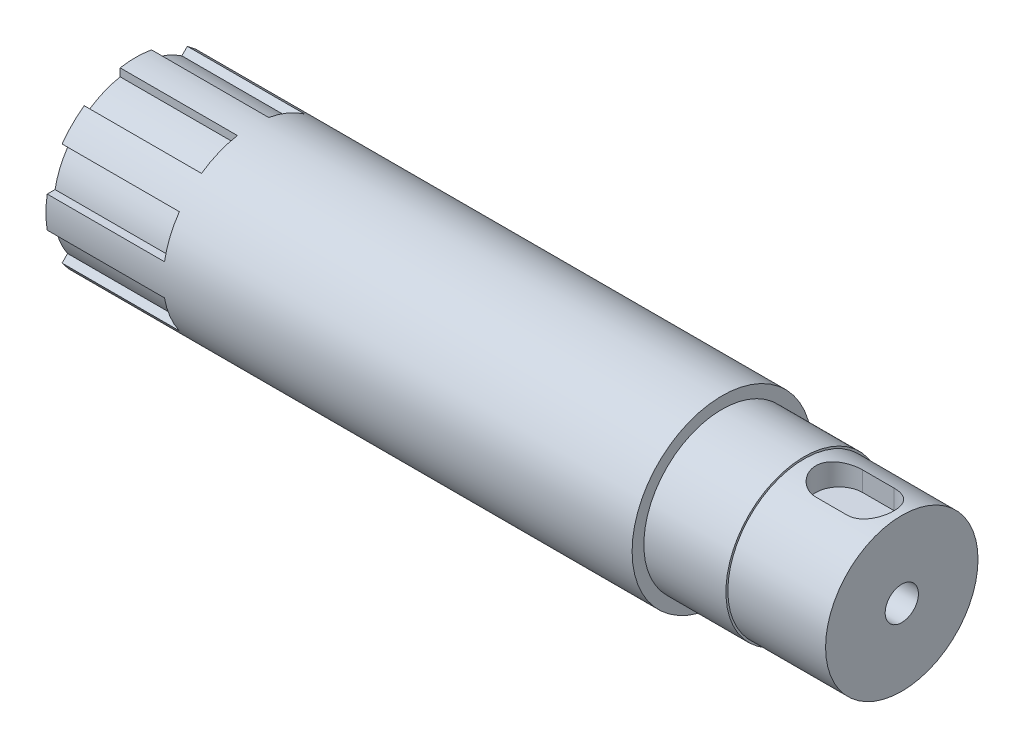
from build123d import *

# Parameters (mm, degrees)
SKETCH_1_R              = 19.5
EXTRUDE_1_DEPTH         = 25
CUT_EXTRUDE_1_DEPTH     = 5.95
SKETCH_3_R              = 20
EXTRUDE_2_DEPTH         = 21
SKETCH_4_R              = 23
EXTRUDE_3_DEPTH         = 150
CUT_EXTRUDE_START       = -30
CUT_EXTRUDE_2_DEPTH     = 30
HOLE_WIZARD_M10_1_D     = 8.5
HOLE_WIZARD_M10_1_DEPTH = 20
HOLE_WIZARD_M10_1_TIP   = 2.553657631


with BuildPart() as part:
    # 草图1 → 凸台-拉伸1 (new body)
    with BuildSketch(Plane(origin=(0, 0, 0), x_dir=(0, 0, -1), z_dir=(1, 0, 0))):
        Circle(SKETCH_1_R)
    extrude(amount=EXTRUDE_1_DEPTH)

    # 草图2 → 切除-拉伸1 (cut)
    with BuildSketch(Plane(origin=(0, 19.5, 0), x_dir=(1, 0, 0), z_dir=(0, 1, 0))):
        with BuildLine():
            Line((9, 6), (17, 6))
            ThreePointArc((17, 6), (23, 0), (17, -6))
            Line((17, -6), (9, -6))
            ThreePointArc((9, -6), (3, 0), (9, 6))
        make_face()
    extrude(amount=-CUT_EXTRUDE_1_DEPTH, mode=Mode.SUBTRACT)

    # 草图3 → 凸台-拉伸2 (add)
    with BuildSketch(Plane.ZY):
        with Locations(Location((0, 0, 0), (0, 0, 180))):
            Circle(SKETCH_3_R)
    extrude(amount=EXTRUDE_2_DEPTH)

    # 草图4 → 凸台-拉伸3 (add)
    with BuildSketch(Plane.ZY.offset(21)):
        Circle(SKETCH_4_R)
    extrude(amount=EXTRUDE_3_DEPTH)

    # 草图5 → 切除-拉伸2 (cut)
    with BuildSketch(Plane.ZY.offset(171).offset(CUT_EXTRUDE_START)):
        with BuildLine():
            ThreePointArc((18.852862485, -13.174580681), (21.255112475, -8.78750213), (22.652173913, -3.98484843))
            Line((22.652173913, -3.98484843), (20.658042319, -3.98484843))
            ThreePointArc((20.658042319, -3.98484843), (19.443275073, -8.036963599), (17.442433123, -11.764151318))
            Line((17.442433123, -11.764151318), (18.852862485, -13.174580681))
        make_face()
        with BuildLine():
            ThreePointArc((22.646822247, 4.01515157), (21.243336512, 8.81593182), (18.83521913, 13.199792435))
            Line((18.83521913, 13.199792435), (17.425155157, 11.789728463))
            ThreePointArc((17.425155157, 11.789728463), (19.431463114, 8.065480192), (20.652173913, 4.01515157))
            Line((20.652173913, 4.01515157), (22.646822247, 4.01515157))
        make_face()
        with BuildLine():
            Line((-20.652173913, -4.01515157), (-22.646822247, -4.01515157))
            ThreePointArc((-22.646822247, -4.01515157), (-21.243336512, -8.81593182), (-18.83521913, -13.199792435))
            Line((-18.83521913, -13.199792435), (-17.425155157, -11.789728463))
            ThreePointArc((-17.425155157, -11.789728463), (-19.431463114, -8.065480192), (-20.652173913, -4.01515157))
        make_face()
        with BuildLine():
            Line((-11.764151318, -17.442433123), (-13.174580681, -18.852862485))
            ThreePointArc((-13.174580681, -18.852862485), (-8.78750213, -21.255112475), (-3.98484843, -22.652173913))
            Line((-3.98484843, -22.652173913), (-3.98484843, -20.658042319))
            ThreePointArc((-3.98484843, -20.658042319), (-8.036963599, -19.443275073), (-11.764151318, -17.442433123))
        make_face()
        with BuildLine():
            ThreePointArc((4.01515157, -22.646822247), (8.81593182, -21.243336512), (13.199792435, -18.83521913))
            Line((13.199792435, -18.83521913), (11.789728463, -17.425155157))
            ThreePointArc((11.789728463, -17.425155157), (8.065480192, -19.431463114), (4.01515157, -20.652173913))
            Line((4.01515157, -20.652173913), (4.01515157, -22.646822247))
        make_face()
        with BuildLine():
            ThreePointArc((13.174580681, 18.852862485), (8.78750213, 21.255112475), (3.98484843, 22.652173913))
            Line((3.98484843, 22.652173913), (3.98484843, 20.658042319))
            ThreePointArc((3.98484843, 20.658042319), (8.036963599, 19.443275073), (11.764151318, 17.442433123))
            Line((11.764151318, 17.442433123), (13.174580681, 18.852862485))
        make_face()
        with BuildLine():
            Line((-4.01515157, 20.652173913), (-4.01515157, 22.646822247))
            ThreePointArc((-4.01515157, 22.646822247), (-8.81593182, 21.243336512), (-13.199792435, 18.83521913))
            Line((-13.199792435, 18.83521913), (-11.789728463, 17.425155157))
            ThreePointArc((-11.789728463, 17.425155157), (-8.065480192, 19.431463114), (-4.01515157, 20.652173913))
        make_face()
        with BuildLine():
            Line((-17.442433123, 11.764151318), (-18.852862485, 13.174580681))
            ThreePointArc((-18.852862485, 13.174580681), (-21.255112475, 8.78750213), (-22.652173913, 3.98484843))
            Line((-22.652173913, 3.98484843), (-20.658042319, 3.98484843))
            ThreePointArc((-20.658042319, 3.98484843), (-19.443275073, 8.036963599), (-17.442433123, 11.764151318))
        make_face()
    extrude(amount=CUT_EXTRUDE_2_DEPTH, mode=Mode.SUBTRACT)

    # M10 螺纹孔1
    with Locations(Plane(origin=(25, 0, 0), x_dir=(0, 0, -1), z_dir=(1, 0, 0))):
        with Locations((0, 0)):
            Hole(HOLE_WIZARD_M10_1_D / 2, depth=HOLE_WIZARD_M10_1_DEPTH)
            with Locations((0, 0, -(HOLE_WIZARD_M10_1_DEPTH + HOLE_WIZARD_M10_1_TIP / 2))):  # 118° drill point
                Cone(0, HOLE_WIZARD_M10_1_D / 2, HOLE_WIZARD_M10_1_TIP, mode=Mode.SUBTRACT)


solid = part.part
